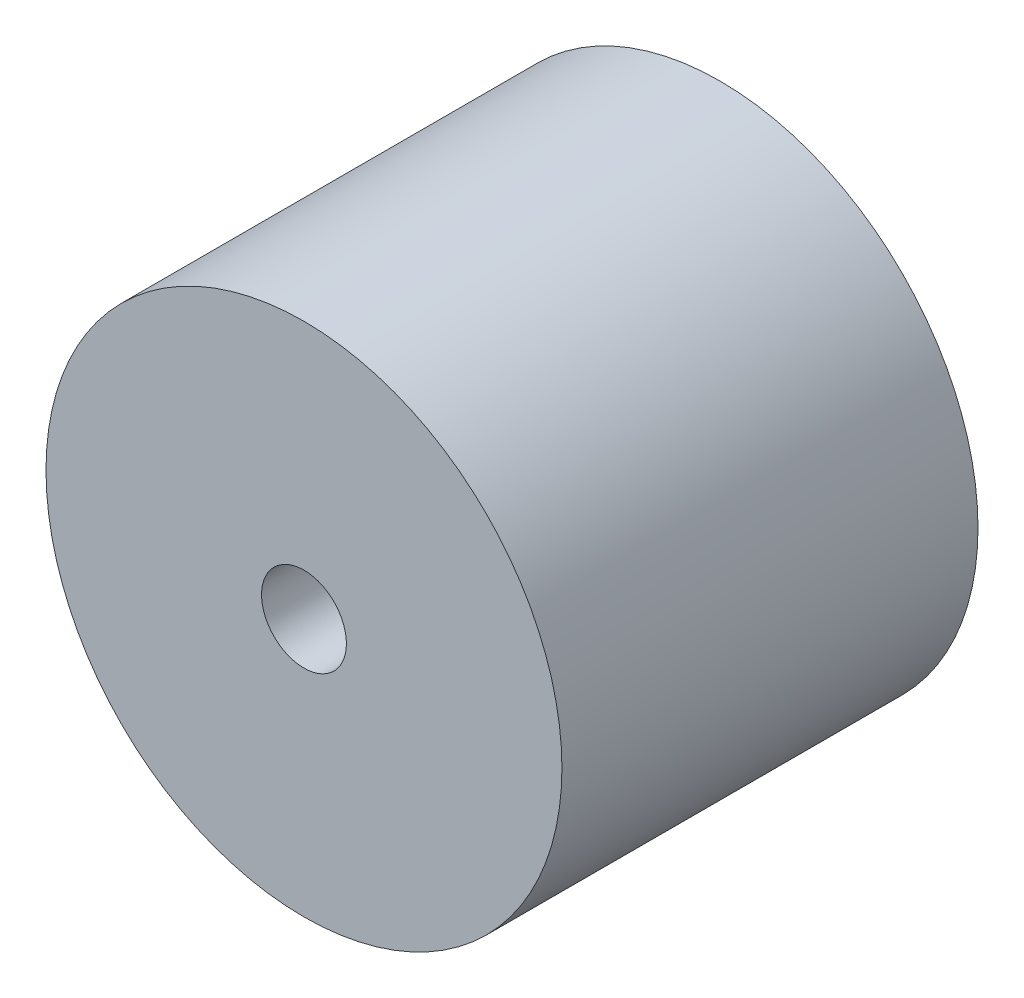
SolidWorks part; units mm, degrees
ref_plane "Front Plane" through (0, 0, 0) normal (0, 0, 1) x (1, 0, 0)
ref_plane "Top Plane" through (0, 0, 0) normal (0, 1, 0) x (1, 0, 0)
ref_plane "Right Plane" through (0, 0, 0) normal (1, 0, 0) x (0, 0, -1)
other "Configuration Table"
sketch "Sketch1" plane through (0, 0, 0) normal (0, 0, 1) x (1, 0, 0)
  circle A0 centre (0, 0) radius 31
extrude "Boss-Extrude1" add sketch "Sketch1" along normal blind 50
sketch "Sketch2" plane through (0, 0, 50) normal (0, 0, 1) x (1, 0, 0)
  circle A0 centre (0, 0) radius 6
hole_wizard "M12 Tapped Hole1" positions "Sketch5" profile "Sketch4" tap size "M12" standard "GB"
sketch "Sketch5" plane through (0, 0, 50) normal (0, 0, 1) x (1, 0, 0)
  point P0 (0, 0)
sketch "Sketch4" plane through (0, 0, 50) normal (1, 0, 0) x (0, -1, 0)
  line L0 (0, 0) -> (0, 32.3144)
  line L1 (0, 32.3144) -> (5.1, 29.25)
  line L2 (5.1, 29.25) -> (5.1, 0)
  line L5 (5.1, 0) -> (0, 0)
  line L10 (0, 32.3144) -> (-5.1, 29.25) construction
  line L11 (0, -6.35) -> (0, 107.95) construction
  dimension "螺纹孔钻头直径" = 10.2
  dimension "螺纹孔钻头深度" = 29.25
  dimension "导头角度" = 118
cosmetic thread "Cosmetic Thread1" parameters "D1"=24, "D2"=12
